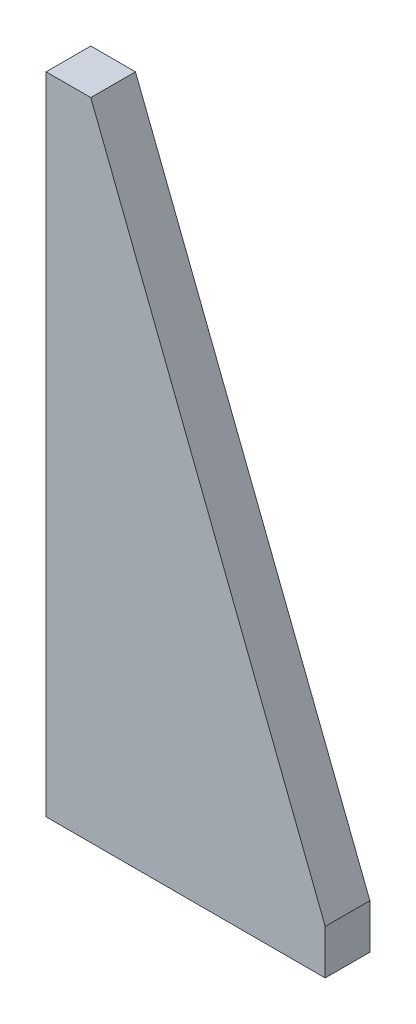
SolidWorks part; units mm, degrees
material "Q235B"
ref_plane "Front Plane" through (0, 0, 0) normal (0, 0, 1) x (1, 0, 0)
ref_plane "Top Plane" through (0, 0, 0) normal (0, 1, 0) x (1, 0, 0)
ref_plane "Right Plane" through (0, 0, 0) normal (1, 0, 0) x (0, 0, -1)
sketch "Sketch1" plane through (0, 0, 0) normal (0, 0, 1) x (1, 0, 0)
  line L0 (0, 0) -> (0, 289)
  line L1 (0, 289) -> (20, 289)
  line L2 (20, 289) -> (125, 20)
  line L3 (125, 20) -> (125, 0)
  line L4 (125, 0) -> (0, 0)
  dimension "D1" = 289
  dimension "D2" = 125
  dimension "D3" = 20
  dimension "D4" = 20
extrude "Boss-Extrude1" add sketch "Sketch1" along normal blind 20
